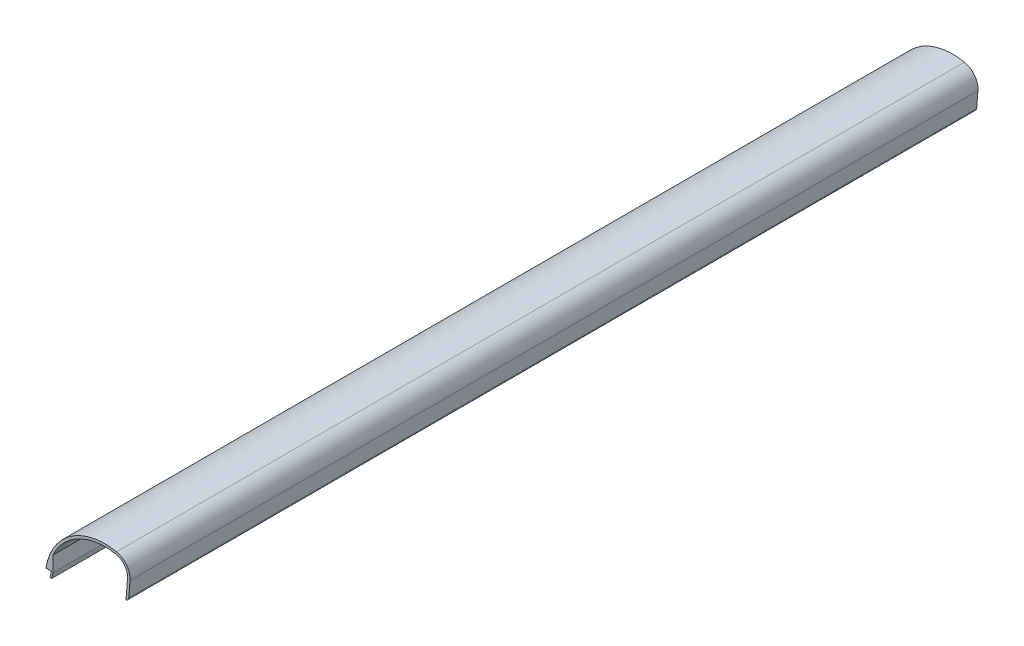
from build123d import *

# Parameters (mm, degrees)
BOSS_EXTRUDE1_DEPTH = 1700
BOSS_EXTRUDE2_START = -30
BOSS_EXTRUDE2_DEPTH = 30
BOSS_EXTRUDE3_DEPTH = 10
BOSS_EXTRUDE4_DEPTH = 30
BOSS_EXTRUDE5_START = -10
SKETCH5_R           = 7.5
BOSS_EXTRUDE5_DEPTH = 10
BOSS_EXTRUDE6_DEPTH = 50
BOSS_EXTRUDE7_DEPTH = 10
BOSS_EXTRUDE8_DEPTH = 10


with BuildPart() as part:
    # Sketch1 → Boss-Extrude1 (new body)
    with BuildSketch(Plane.XY):
        with BuildLine():
            Line((-65.267879059, -3), (-65.267879058, 28.072707798))
            ThreePointArc((-65.267879058, 28.072707798), (-13.334579465, 82.12835912), (60.939776886, 92.247698777))
            ThreePointArc((60.939776886, 92.247698777), (78.362831346, 81.25939595), (84.094528642, 61.474217866))
            Line((84.094528642, 61.474217866), (80.979878482, 23.151827152))
            ThreePointArc((80.979878482, 23.151827152), (84.785028981, 25.375793105), (86.506862858, 29.432945182))
            Line((86.506862858, 29.432945182), (89.078095967, 61.069178711))
            ThreePointArc((89.078095967, 61.069178711), (82.358174999, 84.265594396), (61.931145633, 97.148432192))
            ThreePointArc((61.931145633, 97.148432192), (-30.014942614, 77.922838587), (-79.371264048, -2))
            Line((-79.371264048, -2), (-72.901993076, -2))
            Line((-72.901993076, -2), (-71.577659573, -2))
            Line((-71.577659573, -2), (-68.652793332, -2))
            Line((-68.652793332, -2), (-71.423211626, -14))
            Line((-71.423211626, -14), (-67.807429161, -14))
            Line((-67.807429161, -14), (-65.267879059, -3))
        make_face()
    extrude(amount=-BOSS_EXTRUDE1_DEPTH)

    # Sketch2 → Boss-Extrude2 (add)
    with BuildSketch(Plane(origin=(0, 0, -1290), x_dir=(-1, 0, 0), z_dir=(0, 0, -1)).offset(BOSS_EXTRUDE2_START)):
        with BuildLine():
            Line((-3.532725505, -3), (65.267879058, -3))
            Line((65.267879058, -3), (65.267879058, 28.072707798))
            ThreePointArc((65.267879058, 28.072707798), (13.334579465, 82.12835912), (-60.939776886, 92.247698777))
            ThreePointArc((-60.939776886, 92.247698777), (-78.362831346, 81.25939595), (-84.094528642, 61.474217866))
            Line((-84.094528642, 61.474217866), (-80.979878482, 23.151827152))
            ThreePointArc((-80.979878482, 23.151827152), (-74.905661708, 24.744839622), (-72.552874348, 30.567054818))
            Line((-72.552874348, 30.567054818), (-74.277142478, 51.782303262))
            ThreePointArc((-74.277142478, 51.782303262), (-69.556885099, 65.692259025), (-56.187673771, 71.777642129))
            ThreePointArc((-56.187673771, 71.777642129), (-26.084255804, 61.301829041), (-10.01691723, 33.773678645))
            Line((-10.01691723, 33.773678645), (-3.532725505, -3))
        make_face()
    extrude(amount=BOSS_EXTRUDE2_DEPTH)

    # Sketch3 → Boss-Extrude3 (add)
    with BuildSketch(Plane(origin=(0, 0, -1280), x_dir=(-1, 0, 0), z_dir=(0, 0, -1))):
        with BuildLine():
            Line((55.457231442, -3), (30.270213705, -3))
            ThreePointArc((30.270213705, -3), (36.532321703, -31.272768855), (49.132078223, -57.345927293))
            ThreePointArc((49.132078223, -57.345927293), (65.889976377, -61.288327787), (70.23019688, -44.629031338))
            ThreePointArc((70.23019688, -44.629031338), (60.990271903, -24.472249888), (55.457231442, -3))
        make_face()
        with BuildLine():
            ThreePointArc((52.029725897, -50.736277995), (59.529725897, -58.236277995), (67.029725897, -50.736277995))
            ThreePointArc((67.029725897, -50.736277995), (59.529725897, -43.236277995), (52.029725897, -50.736277995))
        make_face(mode=Mode.SUBTRACT)
    extrude(amount=-BOSS_EXTRUDE3_DEPTH)

    # Sketch4 → Boss-Extrude4 (add)
    with BuildSketch(Plane.XY.offset(-410)):
        with BuildLine():
            Line((3.532725505, -3), (10.01691723, 33.773678645))
            ThreePointArc((10.01691723, 33.773678645), (26.084255804, 61.301829041), (56.187673771, 71.777642129))
            ThreePointArc((56.187673771, 71.777642129), (69.556885099, 65.692259025), (74.277142478, 51.782303262))
            Line((74.277142478, 51.782303262), (72.552874348, 30.567054818))
            ThreePointArc((72.552874348, 30.567054818), (74.905661708, 24.744839622), (80.979878482, 23.151827152))
            Line((80.979878482, 23.151827152), (84.094528642, 61.474217866))
            ThreePointArc((84.094528642, 61.474217866), (78.362831346, 81.25939595), (60.939776886, 92.247698777))
            ThreePointArc((60.939776886, 92.247698777), (-13.334579465, 82.12835912), (-65.267879058, 28.072707798))
            Line((-65.267879058, 28.072707798), (-65.267879058, -3))
            Line((-65.267879058, -3), (3.532725505, -3))
        make_face()
    extrude(amount=-BOSS_EXTRUDE4_DEPTH)

    # Sketch5 → Boss-Extrude5 (add)
    with BuildSketch(Plane.XY.offset(-420).offset(BOSS_EXTRUDE5_START)):
        with BuildLine():
            Line((-30.270213705, -3), (-55.457231442, -3))
            ThreePointArc((-55.457231442, -3), (-60.990271903, -24.472249888), (-70.23019688, -44.629031338))
            ThreePointArc((-70.23019688, -44.629031338), (-65.889976377, -61.288327787), (-49.132078223, -57.345927293))
            ThreePointArc((-49.132078223, -57.345927293), (-36.532321703, -31.272768855), (-30.270213705, -3))
        make_face()
        with Locations(Location((-59.529725897, -50.736277995, 0), (0, 0, 180))):
            Circle(SKETCH5_R, mode=Mode.SUBTRACT)
    extrude(amount=BOSS_EXTRUDE5_DEPTH)

    # Sketch7 → Boss-Extrude6 (add)
    with BuildSketch(Plane.XY.offset(-835)):
        with BuildLine():
            Line((3.532725505, -3), (10.01691723, 33.773678645))
            ThreePointArc((10.01691723, 33.773678645), (26.084255804, 61.301829041), (56.187673771, 71.777642129))
            ThreePointArc((56.187673771, 71.777642129), (69.556885099, 65.692259025), (74.277142478, 51.782303262))
            Line((74.277142478, 51.782303262), (72.552874348, 30.567054818))
            ThreePointArc((72.552874348, 30.567054818), (74.905661708, 24.744839622), (80.979878482, 23.151827152))
            Line((80.979878482, 23.151827152), (84.094528642, 61.474217866))
            ThreePointArc((84.094528642, 61.474217866), (78.362831346, 81.25939595), (60.939776886, 92.247698777))
            ThreePointArc((60.939776886, 92.247698777), (-13.334579465, 82.12835912), (-65.267879058, 28.072707798))
            Line((-65.267879058, 28.072707798), (-65.267879059, -3))
            Line((-65.267879059, -3), (3.532725505, -3))
        make_face()
    extrude(amount=-BOSS_EXTRUDE6_DEPTH)

    # Sketch8 → Boss-Extrude7 (add)
    with BuildSketch(Plane.XY.offset(-845)):
        with BuildLine():
            Line((-22.236687148, -3), (-22.236687148, -17.7))
            ThreePointArc((-22.236687148, -17.7), (-11.738978189, -29.156239028), (0.588602012, -19.696954043))
            Line((0.588602012, -19.696954043), (3.532725505, -3))
            Line((3.532725505, -3), (-22.236687148, -3))
        make_face()
        with BuildLine():
            ThreePointArc((-5.736687148, -17.7), (-10.736687148, -12.7), (-15.736687148, -17.7))
            ThreePointArc((-15.736687148, -17.7), (-10.736687148, -22.7), (-5.736687148, -17.7))
        make_face(mode=Mode.SUBTRACT)
    extrude(amount=-BOSS_EXTRUDE7_DEPTH)

    # Sketch9 → Boss-Extrude8 (add)
    with BuildSketch(Plane.XY.offset(-865)):
        with BuildLine():
            Line((-22.236687148, -3), (-22.236687148, -17.699999999))
            ThreePointArc((-22.236687148, -17.699999999), (-11.73897819, -29.156239028), (0.588602012, -19.696954043))
            Line((0.588602012, -19.696954043), (3.532725505, -3))
            Line((3.532725505, -3), (-22.236687148, -3))
        make_face()
        with BuildLine():
            ThreePointArc((-5.736687148, -17.7), (-10.736687148, -12.7), (-15.736687148, -17.7))
            ThreePointArc((-15.736687148, -17.7), (-10.736687148, -22.7), (-5.736687148, -17.7))
        make_face(mode=Mode.SUBTRACT)
    extrude(amount=-BOSS_EXTRUDE8_DEPTH)


solid = part.part
